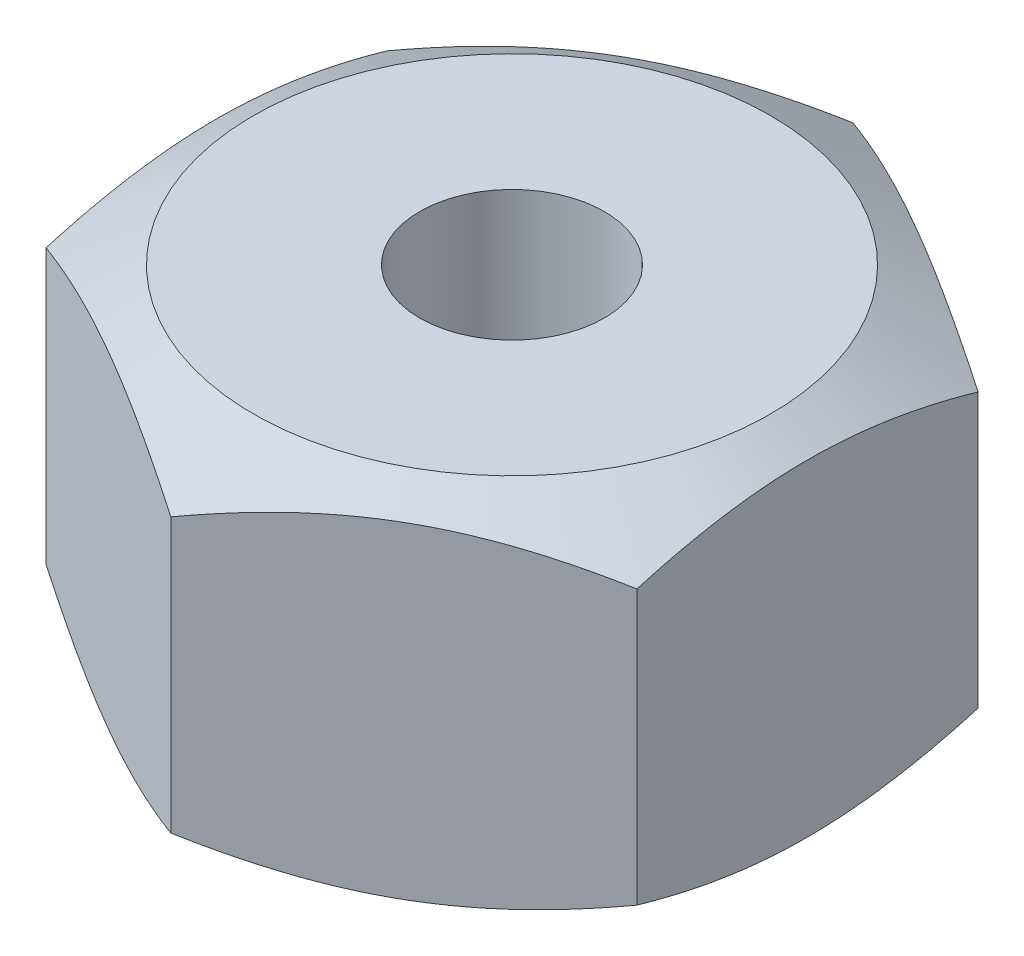
from build123d import *

# Parameters (mm, degrees)
BOSS_EXTRUDE1_DEPTH = 10
SKETCH2_R           = 5
CUT_EXTRUDE1_DEPTH  = 50
CUT_EXTRUDE2_START  = -15
SKETCH3_R           = 14
CUT_EXTRUDE2_DEPTH  = 4


with BuildPart() as part:
    # Sketch1 → Boss-Extrude1 (new, symmetric)
    with BuildSketch(Plane(origin=(0, 0, 0), x_dir=(1, 0, 0), z_dir=(0, 1, 0))):
        Polygon((0, 18.475208614), (-16, 9.237604307), (-16, -9.237604307), (0, -18.475208614), (16, -9.237604307), (16, 9.237604307), align=None)
    extrude(amount=BOSS_EXTRUDE1_DEPTH, both=True)

    # Sketch2 → Cut-Extrude1 (cut)
    with BuildSketch(Plane(origin=(0, 10, 0), x_dir=(1, 0, 0), z_dir=(0, 1, 0))):
        with Locations(Location((0, 0, 0), (0, 0, 270))):
            Circle(SKETCH2_R)
    extrude(amount=-CUT_EXTRUDE1_DEPTH, mode=Mode.SUBTRACT)

    # Sketch3 → Cut-Extrude2 (cut)
    with BuildSketch(Plane(origin=(0, 10, 0), x_dir=(1, 0, 0), z_dir=(0, 1, 0)).offset(CUT_EXTRUDE2_START)):
        with Locations(Location((0, 0, 0), (0, 0, 270))):
            Circle(SKETCH3_R)
    extrude(amount=CUT_EXTRUDE2_DEPTH, mode=Mode.SUBTRACT)

    # Sketch4 → Cut-Revolve1 (revolve, cut)
    with BuildSketch(Plane(origin=(0, 0, 0), x_dir=(0, 0, -1), z_dir=(1, 0, 0))):
        Polygon((18.475208614, 7.416237102), (18.475208614, 10), (14, 10), align=None)
    cut_revolve1 = revolve(axis=Axis((0, 0, 0), (0, 1, 0)), mode=Mode.SUBTRACT)

    # Mirror1: Cut-Revolve1 across plane
    add(cut_revolve1.mirror(Plane.ZX), mode=Mode.SUBTRACT)


solid = part.part
